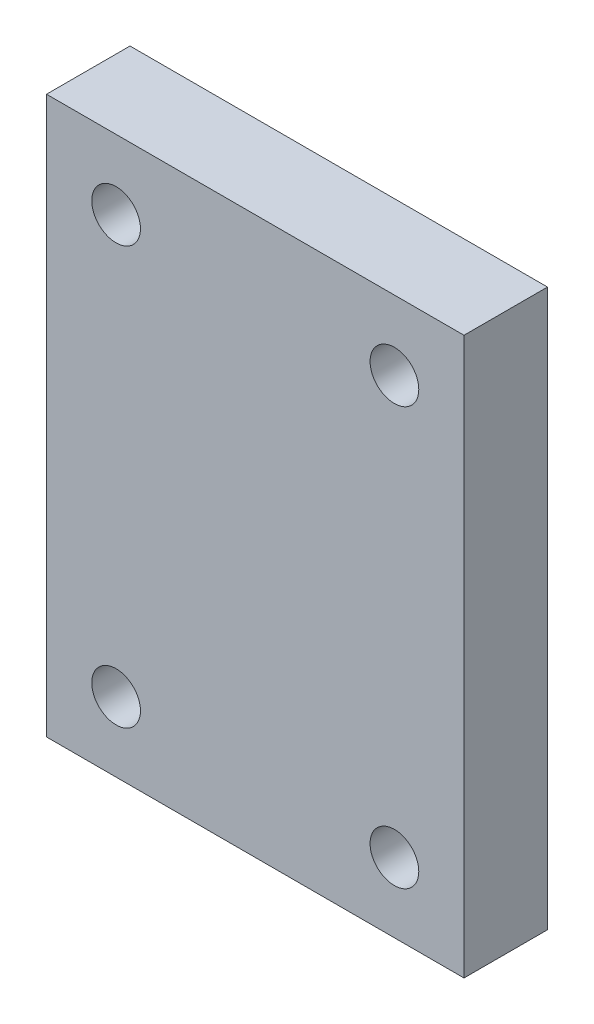
from build123d import *

# Parameters (mm, degrees)
SKETCH1_W            = 150
SKETCH1_H            = 200
BOSS_EXTRUDE1_DEPTH  = 30
M20_THREADED_HOLE1_D = 17.5


with BuildPart() as part:
    # Sketch1 → Boss-Extrude1 (new body)
    with BuildSketch(Plane.XY):
        with Locations((75, 100)):
            Rectangle(SKETCH1_W, SKETCH1_H)
    extrude(amount=BOSS_EXTRUDE1_DEPTH)

    # M20 Threaded hole1 (through all)
    with Locations(Plane(origin=(25, 175, 30), x_dir=(1, 0, 0), z_dir=(0, 0, 1))):
        with Locations((0, 0), (100, 0), (0, -150), (100, -150)):
            Hole(M20_THREADED_HOLE1_D / 2)


solid = part.part
